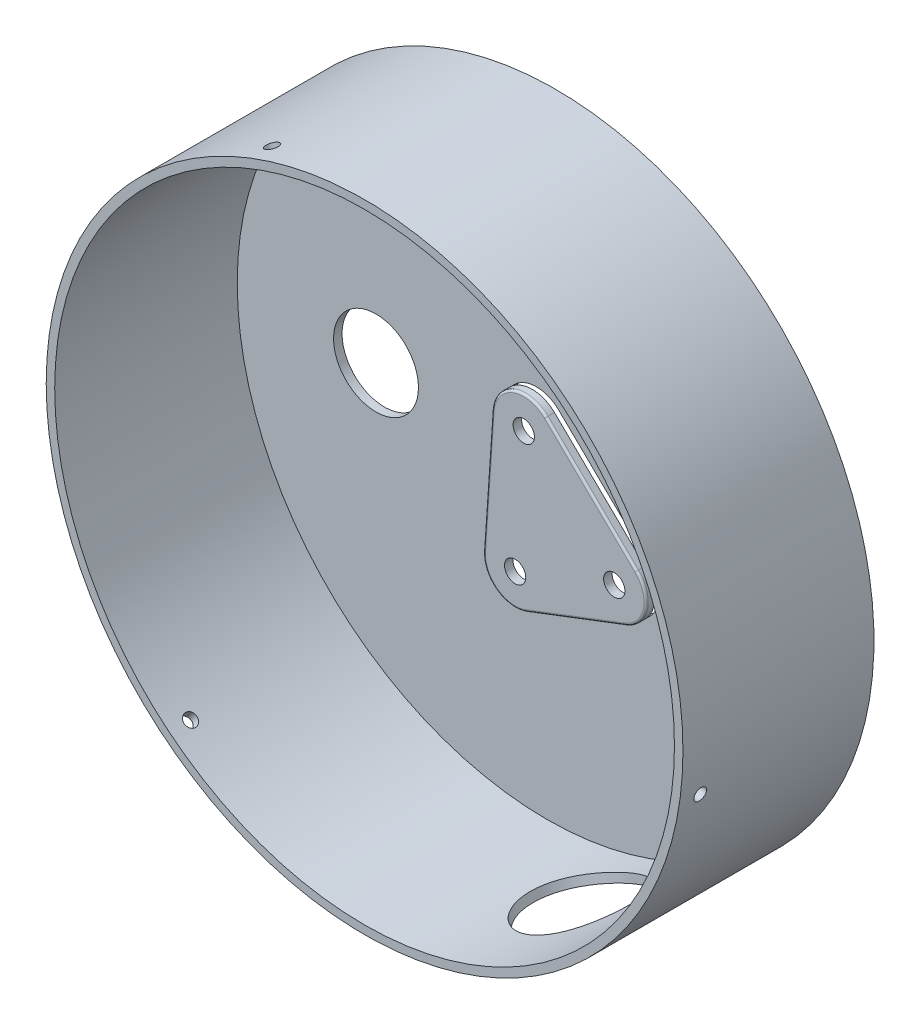
from build123d import *

# Parameters (mm, degrees)
SKETCH_1_R                = 75
SKETCH_1_R_2              = 73
BOSS_EXTRUDE_1_DEPTH      = 48
SKETCH_2_R                = 75
BOSS_EXTRUDE_2_DEPTH      = 5
SKETCH_4_R                = 10
CUT_EXTRUDE_8_DEPTH       = 117.421647472
SKETCH_8_R                = 75
CUT_EXTRUDE_10_DEPTH      = 3
CUT_EXTRUDE_12_REACH      = 185.592
CUT_EXTRUDE_12_END_RADIUS = 73
SKETCH_11_R               = 12.5
SKETCH_20_R               = 2.5
CUT_EXTRUDE_19_DEPTH      = 117.421647642
SKETCH_21_R               = 2.5
BOSS_EXTRUDE_3_DEPTH      = 3
CUT_EXTRUDE_21_DEPTH      = 6
FILLET_2_R                = 0.5
CUT_EXTRUDE_22_REACH      = 185.592
CUT_EXTRUDE_22_END_RADIUS = 73
SKETCH_24_R               = 1.5
CIRCULAR_PATTERN_1_COUNT  = 3


with BuildPart() as part:
    # Sketch 1 → Boss-Extrude 1 (new body)
    with BuildSketch(Plane.XY):
        Circle(SKETCH_1_R)
        Circle(SKETCH_1_R_2, mode=Mode.SUBTRACT)
    extrude(amount=BOSS_EXTRUDE_1_DEPTH)

    # Sketch 2 → Boss-Extrude 2 (add)
    with BuildSketch(Plane.XY):
        Circle(SKETCH_2_R)
    extrude(amount=BOSS_EXTRUDE_2_DEPTH)

    # Sketch 4 → Cut-Extrude 8 (cut, through all)
    with BuildSketch(Plane.XY):
        with Locations((-40.31, 0)):
            Circle(SKETCH_4_R)
    extrude(amount=CUT_EXTRUDE_8_DEPTH, mode=Mode.SUBTRACT)

    # Sketch 8 → Cut-Extrude 10 (cut)
    with BuildSketch(Plane(origin=(0, 0, 0), x_dir=(-1, 0, 0), z_dir=(0, 0, -1))):
        Circle(SKETCH_8_R)
        with BuildLine():
            Line((12.012248906, -22.631496582), (9.983760796, 7.049267155))
            ThreePointArc((9.983760796, 7.049267155), (5.18108887, 13.542758882), (-2.729335581, 11.912949859))
            Line((-2.729335581, 11.912949859), (-24.05043175, -8.834902033))
            ThreePointArc((-24.05043175, -8.834902033), (-26.165589934, -15.723427277), (-21.499754406, -21.214843578))
            Line((-21.499754406, -21.214843578), (1.849829873, -30.147755422))
            ThreePointArc((1.849829873, -30.147755422), (8.989518573, -29.172809562), (12.012248906, -22.631496582))
        make_face(mode=Mode.SUBTRACT)
    extrude(amount=-CUT_EXTRUDE_10_DEPTH, mode=Mode.SUBTRACT)

    # Cut-Extrude 12: up to this cylinder (the profile starts outside it)
    cut_extrude_12_end = Plane(origin=(0, 0, 23), z_dir=(0, 0, -1)) * Cylinder(CUT_EXTRUDE_12_END_RADIUS, 518.184, mode=Mode.PRIVATE)
    # Sketch 11 → Cut-Extrude 12 (cut, up to the surface)
    with BuildSketch(Plane(origin=(26.798735532, -70.048752836, 0), x_dir=(-0.9339833711458582, -0.35731647376383047, 0), z_dir=(0.35731647376383047, -0.9339833711458583, 0)), mode=Mode.PRIVATE) as cut_extrude_12_sk1:
        with Locations(Location((0, -23, 0), (0, 0, 180))):
            Circle(SKETCH_11_R)
    cut_extrude_12_tool1 = extrude(cut_extrude_12_sk1.sketch, amount=-CUT_EXTRUDE_12_REACH, mode=Mode.PRIVATE) - cut_extrude_12_end
    add(cut_extrude_12_tool1.solids().sort_by_distance((26.798736, -70.048753, 23))[0], mode=Mode.SUBTRACT)

    # Sketch 20 → Cut-Extrude 19 (cut, through all)
    with BuildSketch(Plane(origin=(0, 0, 0), x_dir=(-1, 0, 0), z_dir=(0, 0, -1))):
        with Locations((2.501215316, 6.537883598)):
            Circle(SKETCH_20_R)
        with Locations((4.529703426, -23.142880139)):
            Circle(SKETCH_20_R)
        with Locations((-18.819880853, -14.209968294)):
            Circle(SKETCH_20_R)
    extrude(amount=-CUT_EXTRUDE_19_DEPTH, mode=Mode.SUBTRACT)

    # Sketch 21 → Boss-Extrude 3 (add)
    with BuildSketch(Plane.XY.offset(5)):
        with BuildLine():
            Line((24.05043175, -8.834902033), (2.729335581, 11.912949859))
            ThreePointArc((2.729335581, 11.912949859), (-5.18108887, 13.542758882), (-9.983760796, 7.049267155))
            Line((-9.983760796, 7.049267155), (-12.012248906, -22.631496582))
            ThreePointArc((-12.012248906, -22.631496582), (-8.989518573, -29.172809562), (-1.849829873, -30.147755422))
            Line((-1.849829873, -30.147755422), (21.499754406, -21.214843578))
            ThreePointArc((21.499754406, -21.214843578), (26.165589934, -15.723427277), (24.05043175, -8.834902033))
        make_face()
        with Locations(Location((-4.529703426, -23.142880139, 0), (0, 0, 180))):
            Circle(SKETCH_21_R, mode=Mode.SUBTRACT)
        with Locations(Location((18.819880853, -14.209968294, 0), (0, 0, 180))):
            Circle(SKETCH_21_R, mode=Mode.SUBTRACT)
        with Locations(Location((-2.501215316, 6.537883598, 0), (0, 0, 180))):
            Circle(SKETCH_21_R, mode=Mode.SUBTRACT)
    extrude(amount=BOSS_EXTRUDE_3_DEPTH)

    # Sketch 22 → Cut-Extrude 21 (cut)
    with BuildSketch(Plane(origin=(0, 0, 0), x_dir=(-1, 0, 0), z_dir=(0, 0, -1))):
        with BuildLine():
            Line((-2.729335581, 11.912949859), (-24.05043175, -8.834902033))
            ThreePointArc((-24.05043175, -8.834902033), (-26.165589934, -15.723427277), (-21.499754406, -21.214843578))
            Line((-21.499754406, -21.214843578), (1.849829873, -30.147755422))
            ThreePointArc((1.849829873, -30.147755422), (8.989518573, -29.172809562), (12.012248906, -22.631496582))
            Line((12.012248906, -22.631496582), (9.983760796, 7.049267155))
            ThreePointArc((9.983760796, 7.049267155), (5.18108887, 13.542758882), (-2.729335581, 11.912949859))
        make_face()
    extrude(amount=-CUT_EXTRUDE_21_DEPTH, mode=Mode.SUBTRACT)


with BuildPart() as cut_extrude_21_piece_1:
    # of the separate pieces the step leaves, piece 1, a body of its own (cut_extrude_21_pieces)
    add(part.part.solids().sort_by_distance((75, 0, 48))[0])

    # Cut-Extrude 22: up to this cylinder (the profile starts outside it)
    cut_extrude_22_end = Plane(origin=(0, 0, 43), z_dir=(0, 0, -1)) * Cylinder(CUT_EXTRUDE_22_END_RADIUS, 518.184, mode=Mode.PRIVATE)
    # Sketch 24 → Cut-Extrude 22 (cut, up to the surface)
    with BuildSketch(Plane(origin=(-26.798735532, 70.048752836, 0), x_dir=(0.9339833711458588, 0.3573164737638288, 0), z_dir=(-0.3573164737638288, 0.9339833711458588, 0)), mode=Mode.PRIVATE) as cut_extrude_22_sk1:
        with Locations(Location((0, -43, 0), (0, 0, 180))):
            Circle(SKETCH_24_R)
    cut_extrude_22_tool1 = extrude(cut_extrude_22_sk1.sketch, amount=-CUT_EXTRUDE_22_REACH, mode=Mode.PRIVATE) - cut_extrude_22_end
    cut_extrude_22 = cut_extrude_22_tool1.solids().sort_by_distance((-26.798736, 70.048753, 43))[0]
    add(cut_extrude_22, mode=Mode.SUBTRACT)

    # Circular pattern 1: Cut-Extrude 22 ×3 about axis
    circular_pattern_1_axis = Axis((0, 0, 0), (0, 0, 1))
    for i in range(1, CIRCULAR_PATTERN_1_COUNT):
        add(cut_extrude_22.rotate(circular_pattern_1_axis, i * 360 / CIRCULAR_PATTERN_1_COUNT), mode=Mode.SUBTRACT)


with BuildPart() as cut_extrude_21_piece_2:
    # of the separate pieces the step leaves, piece 2, a body of its own (cut_extrude_21_pieces)
    add(part.part.solids().sort_by_distance((-1.849829873, -30.147755422, 6))[0])

    # Fillet 2
    fillet_2_edges = [cut_extrude_21_piece_2.edges().sort_by_distance(p)[0] for p in [
        (13.389883665, 1.539023913, 8),
        (-5.18108887, 13.542758882, 8),
        (-10.998004851, -7.791114713, 8),
        (-8.989518573, -29.172809562, 8),
        (9.824962267, -25.6812995, 8),
        (26.165589934, -15.723427277, 8),
    ]]
    fillet(fillet_2_edges, radius=FILLET_2_R)


solid = Compound([cut_extrude_21_piece_1.part, cut_extrude_21_piece_2.part])
